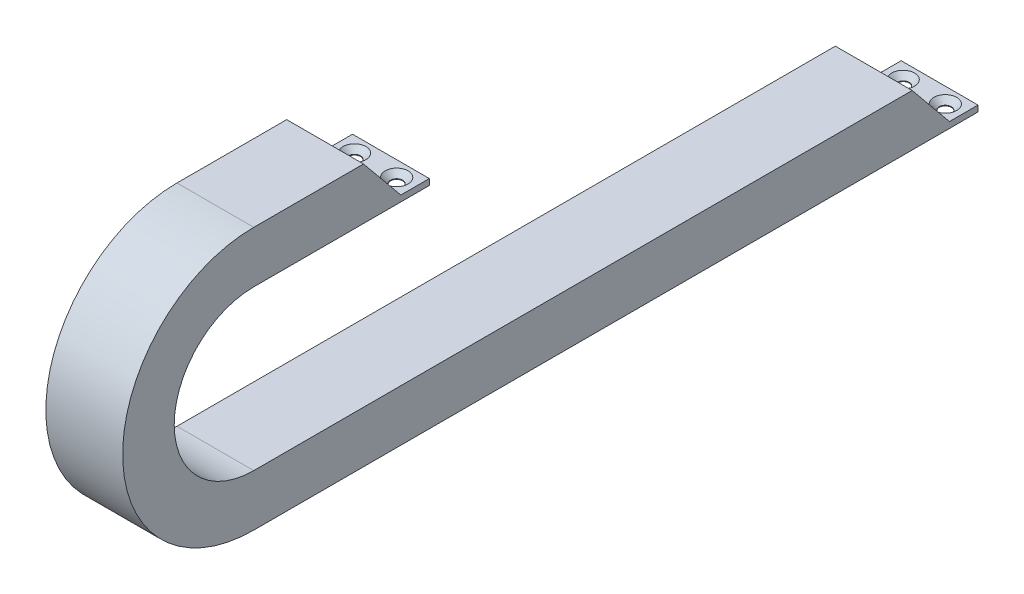
from build123d import *

# Parameters (mm, degrees)
SECTION_SIZE_W                              = 35
SECTION_SIZE_H                              = 23.5
SECTION_SIZE_W_2                            = 25
SECTION_SIZE_H_2                            = 18
SKETCH2_W                                   = 35
SKETCH2_H                                   = 30
FITTING114_4_12PZ_1_DEPTH                   = 2.75
SKETCH6_W                                   = 35
SKETCH6_H                                   = 30
FITTING114_4_12PZ_2_DEPTH                   = 2.75
RIB_E_REACH                                 = 379.167
SKETCH9_WALL_W                              = 783.159137046
SKETCH9_WALL_H                              = 4.1
RIB_Z_REACH                                 = 379.167
SKETCH10_WALL_W                             = 783.159137046
SKETCH10_WALL_H                             = 4.1
M5_FLAT_HEAD_SCREW_COUNTERSINK1_AT_2_COUNT  = 2
M5_FLAT_HEAD_SCREW_COUNTERSINK1_AT_2_PITCH  = 13.862178761
M5_FLAT_HEAD_SCREW_COUNTERSINK1_AT_3_COUNT  = 2
M5_FLAT_HEAD_SCREW_COUNTERSINK1_AT_3_PITCH  = 19.2
M5_FLAT_HEAD_SCREW_COUNTERSINK2_D           = 5.5
M5_FLAT_HEAD_SCREW_COUNTERSINK2_DEPTH       = 35
M5_FLAT_HEAD_SCREW_COUNTERSINK2_CSINK_D     = 10.4
M5_FLAT_HEAD_SCREW_COUNTERSINK2_CSINK_ANGLE = 90
M5_FLAT_HEAD_SCREW_COUNTERSINK2_TIP         = 1.652366702


with BuildPart() as part:
    # Chain: sweep along a path in Length Path
    with BuildLine(Plane(origin=(0, 0, 0), x_dir=(0, 0, -1), z_dir=(1, 0, 0))) as chain_path:
        Line((-250, 96), (-300, 96))
        ThreePointArc((-300, 96), (-348, 48), (-300, 0))
        Line((-300, 0), (0, 0))
    # Section Size → Chain (sweep)
    with BuildSketch(Plane.XY):
        Rectangle(SECTION_SIZE_W, SECTION_SIZE_H)
        Rectangle(SECTION_SIZE_W_2, SECTION_SIZE_H_2, mode=Mode.SUBTRACT)
    sweep(path=chain_path.line)

    # Sketch2 → Fitting114.4.12PZ-1 (add)
    with BuildSketch(Plane(origin=(0, 84.25, 0), x_dir=(1, 0, 0), z_dir=(0, 1, 0))):
        with Locations((0, -235)):
            Rectangle(SKETCH2_W, SKETCH2_H)
    extrude(amount=FITTING114_4_12PZ_1_DEPTH)

    # Sketch6 → Fitting114.4.12PZ-2 (add)
    with BuildSketch(Plane.XZ.offset(11.75)):
        with Locations((0, -15)):
            Rectangle(SKETCH6_W, SKETCH6_H)
    extrude(amount=-FITTING114_4_12PZ_2_DEPTH)

    # Sketch9 wall → E (add, up to next)
    with BuildSketch(Plane(origin=(17.5, 97.375, 241.5), x_dir=(0, -0.773541895, -0.633745166988), z_dir=(0, 0.633745166988, -0.773541895)), mode=Mode.PRIVATE) as rib_e_sk1:
        with Locations((0, 2.05)):
            Rectangle(SKETCH9_WALL_W, SKETCH9_WALL_H)
    rib_e_tool1 = extrude(rib_e_sk1.sketch, amount=-RIB_E_REACH, mode=Mode.PRIVATE) - part.part
    rib_e = rib_e_tool1.solids().sort_by_distance((17.5, 97.375, 241.5))[0]
    add(rib_e)

    # Sketch10 wall → Z (add, up to next)
    with BuildSketch(Plane(origin=(17.5, 1.375, -8.5), x_dir=(0, 0.773541895, 0.633745166988), z_dir=(0, -0.633745166988, 0.773541895)), mode=Mode.PRIVATE) as rib_z_sk1:
        with Locations((0, 2.05)):
            Rectangle(SKETCH10_WALL_W, SKETCH10_WALL_H)
    rib_z_tool1 = extrude(rib_z_sk1.sketch, amount=RIB_Z_REACH, mode=Mode.PRIVATE) - part.part
    rib_z = rib_z_tool1.solids().sort_by_distance((17.5, 1.375, -8.5))[0]
    add(rib_z)

    # Drag: E, Z across plane
    add(rib_e.mirror(Plane(origin=(0, 0, 0), x_dir=(0, 0, 1), z_dir=(1, 0, 0))))
    add(rib_z.mirror(Plane(origin=(0, 0, 0), x_dir=(0, 0, 1), z_dir=(1, 0, 0))))

    # Sketch17 → M5 Flat Head Screw Countersink1 (revolve, cut)
    with BuildSketch(Plane(origin=(-9.6, -9, -23), x_dir=(0, 0, 1), z_dir=(1, 0, 0))):
        Polygon((0, 0), (0, 2.75), (2.75, 2.75), (2.75, 2.45), (5.2, 0), align=None)
    m5_flat_head_screw_countersink1 = revolve(axis=Axis((-9.6, -2.65, -23), (0, -1, 0)), mode=Mode.SUBTRACT)

    # M5 Flat Head Screw Countersink1 at 2: M5 Flat Head Screw Countersink1 ×2
    with Locations(*[Vector(0.6925318281897137, 0, 0.7213873210309515) * (i * M5_FLAT_HEAD_SCREW_COUNTERSINK1_AT_2_PITCH) for i in range(1, M5_FLAT_HEAD_SCREW_COUNTERSINK1_AT_2_COUNT)]):
        add(m5_flat_head_screw_countersink1, mode=Mode.SUBTRACT)

    # M5 Flat Head Screw Countersink1 at 3: M5 Flat Head Screw Countersink1 ×2
    with Locations(*[(i * M5_FLAT_HEAD_SCREW_COUNTERSINK1_AT_3_PITCH, 0, 0) for i in range(1, M5_FLAT_HEAD_SCREW_COUNTERSINK1_AT_3_COUNT)]):
        add(m5_flat_head_screw_countersink1, mode=Mode.SUBTRACT)

    # M5 Flat Head Screw Countersink2
    with Locations(Plane(origin=(-9.6, 87, 227), x_dir=(0, 0, 1), z_dir=(0, 1, 0))):
        with Locations((0, 0), (10, 9.6), (0, 19.2)):
            CounterSinkHole(M5_FLAT_HEAD_SCREW_COUNTERSINK2_D / 2, M5_FLAT_HEAD_SCREW_COUNTERSINK2_CSINK_D / 2, depth=M5_FLAT_HEAD_SCREW_COUNTERSINK2_DEPTH, counter_sink_angle=M5_FLAT_HEAD_SCREW_COUNTERSINK2_CSINK_ANGLE)
            with Locations((0, 0, -(M5_FLAT_HEAD_SCREW_COUNTERSINK2_DEPTH + M5_FLAT_HEAD_SCREW_COUNTERSINK2_TIP / 2))):  # 118° drill point
                Cone(0, M5_FLAT_HEAD_SCREW_COUNTERSINK2_D / 2, M5_FLAT_HEAD_SCREW_COUNTERSINK2_TIP, mode=Mode.SUBTRACT)


solid = part.part
